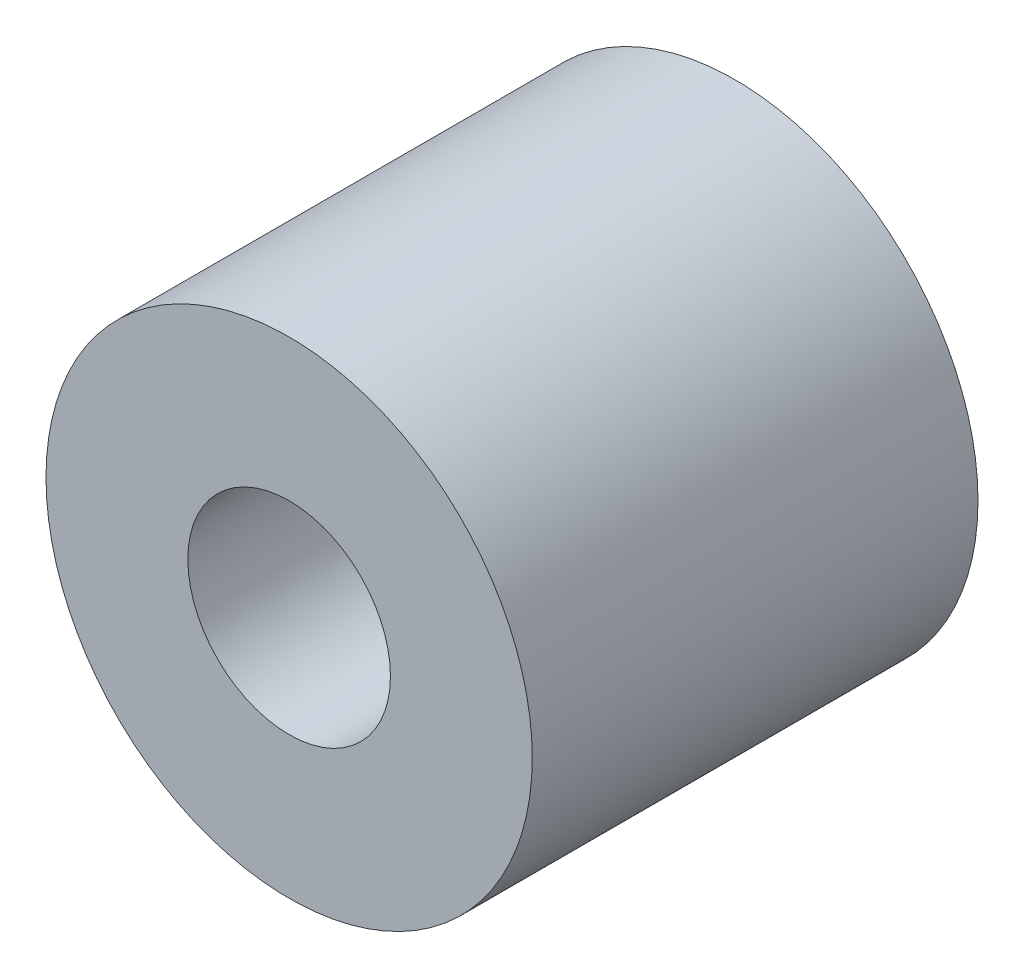
SolidWorks part; units mm, degrees
ref_plane "前视基准面" through (0, 0, 0) normal (0, 0, 1) x (1, 0, 0)
ref_plane "上视基准面" through (0, 0, 0) normal (0, 1, 0) x (1, 0, 0)
ref_plane "右视基准面" through (0, 0, 0) normal (1, 0, 0) x (0, 0, -1)
other "Configuration Table"
sketch "草图1" plane through (0, 0, 0) normal (0, 0, 1) x (1, 0, 0)
  circle A0 centre (0, 0) radius 3
  circle A1 centre (0, 0) radius 1.25
  point P0 (0, 0)
  dimension "D1" = 2.5
  dimension "D2" = 6
extrude "凸台-拉伸1" add sketch "草图1" against normal mid plane 5.5
